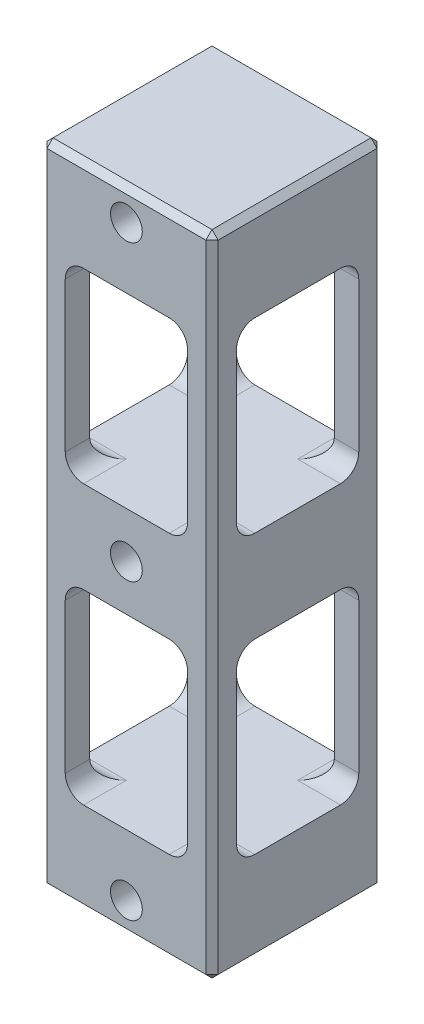
SolidWorks part; units mm, degrees
material "ABS"
ref_plane "前视基准面" through (0, 0, 0) normal (0, 0, 1) x (1, 0, 0)
ref_plane "上视基准面" through (0, 0, 0) normal (0, 1, 0) x (1, 0, 0)
ref_plane "右视基准面" through (0, 0, 0) normal (1, 0, 0) x (0, 0, -1)
other "Configuration Table"
sketch "草图1" plane through (0, 0, 0) normal (0, 1, 0) x (1, 0, 0)
  line L1 (-14, -14) -> (14, -14)
  line L2 (-14, -14) -> (-14, 14)
  line L3 (-14, 14) -> (14, 14)
  line L4 (14, -14) -> (14, 14)
  line L5 (-14, -14) -> (14, 14) construction
  line L6 (-14, 14) -> (14, -14) construction
  point P0 (0, 0)
  dimension "D1" = 28
extrude "凸台-拉伸1" add sketch "草图1" along normal blind 106
sketch "草图2" plane through (0, 0, 14) normal (0, 0, 1) x (1, 0, 0)
  line L0 (-14, 0) -> (14, 0) construction
  line L1 (-7, 60.5) -> (7, 60.5)
  line L2 (-10, 63.5) -> (-10, 88)
  line L3 (-7, 91) -> (7, 91)
  line L4 (10, 63.5) -> (10, 88)
  line L5 (-10, 60.5) -> (10, 91) construction
  line L6 (-10, 91) -> (10, 60.5) construction
  line L7 (-7, 15) -> (7, 15)
  line L8 (-10, 18) -> (-10, 42.5)
  line L9 (-7, 45.5) -> (7, 45.5)
  line L10 (10, 18) -> (10, 42.5)
  line L11 (-10, 15) -> (10, 45.5) construction
  line L12 (-10, 45.5) -> (10, 15) construction
  line L13 (-14, 106) -> (14, 106) construction
  line L14 (-14, 106) -> (-14, 0) construction
  line L15 (-14, 106) -> (-14, 0) construction
  arc A0 (7, 15) -> (10, 18) centre (7, 18) ccw
  arc A1 (-10, 42.5) -> (-7, 45.5) centre (-7, 42.5) cw
  arc A2 (-7, 15) -> (-10, 18) centre (-7, 18) cw
  arc A3 (7, 45.5) -> (10, 42.5) centre (7, 42.5) cw
  arc A4 (7, 60.5) -> (10, 63.5) centre (7, 63.5) ccw
  arc A5 (-10, 88) -> (-7, 91) centre (-7, 88) cw
  arc A6 (-7, 60.5) -> (-10, 63.5) centre (-7, 63.5) cw
  arc A7 (7, 91) -> (10, 88) centre (7, 88) cw
  circle A8 centre (0, 101) radius 2.6
  circle A9 centre (0, 53) radius 2.6
  circle A10 centre (0, 5) radius 2.6
  point P0 (0, 75.75)
  point P5 (0, 30.25)
  point P47 (-14, 53)
  dimension "D5" = 3
  dimension "D6" = 5.2
  dimension "D1" = 20
  dimension "D2" = 15
  dimension "D3" = 15
  dimension "D4" = 15
  dimension "D7" = 96
  dimension "D8" = 5
extrude "切除-拉伸1" cut sketch "草图2" against normal through all
sketch "草图3" plane through (14, 0, 0) normal (1, 0, 0) x (0, 0, -1)
  line L0 (-14, 0) -> (14, 0) construction
  line L1 (-7, 60.5) -> (7, 60.5)
  line L2 (-10, 63.5) -> (-10, 88)
  line L3 (-7, 91) -> (7, 91)
  line L4 (10, 63.5) -> (10, 88)
  line L5 (-10, 60.5) -> (10, 91) construction
  line L6 (-10, 91) -> (10, 60.5) construction
  line L7 (-7, 15) -> (7, 15)
  line L8 (-10, 18) -> (-10, 42.5)
  line L9 (-7, 45.5) -> (7, 45.5)
  line L10 (10, 18) -> (10, 42.5)
  line L11 (-10, 15) -> (10, 45.5) construction
  line L12 (-10, 45.5) -> (10, 15) construction
  line L13 (-14, 106) -> (14, 106) construction
  arc A0 (7, 15) -> (10, 18) centre (7, 18) ccw
  arc A1 (-10, 42.5) -> (-7, 45.5) centre (-7, 42.5) cw
  arc A2 (-7, 15) -> (-10, 18) centre (-7, 18) cw
  arc A3 (7, 45.5) -> (10, 42.5) centre (7, 42.5) cw
  arc A4 (7, 60.5) -> (10, 63.5) centre (7, 63.5) ccw
  arc A5 (-10, 88) -> (-7, 91) centre (-7, 88) cw
  arc A6 (-7, 60.5) -> (-10, 63.5) centre (-7, 63.5) cw
  arc A7 (7, 91) -> (10, 88) centre (7, 88) cw
  point P0 (0, 75.75)
  point P5 (0, 30.25)
  dimension "D5" = 3
  dimension "D1" = 15
  dimension "D2" = 15
  dimension "D3" = 15
  dimension "D4" = 20
extrude "切除-拉伸2" cut sketch "草图3" against normal through all
chamfer "倒角1" distance 1 angle 45 12 edges at (14, 0, 0) (0, 0, -14) (-14, 0, 0) (0, 0, 14) (14, 106, 0) (14, 53, -14) (0, 106, -14) (-14, 53, -14) (-14, 106, 0) (14, 53, 14) (0, 106, 14) (-14, 53, 14)
